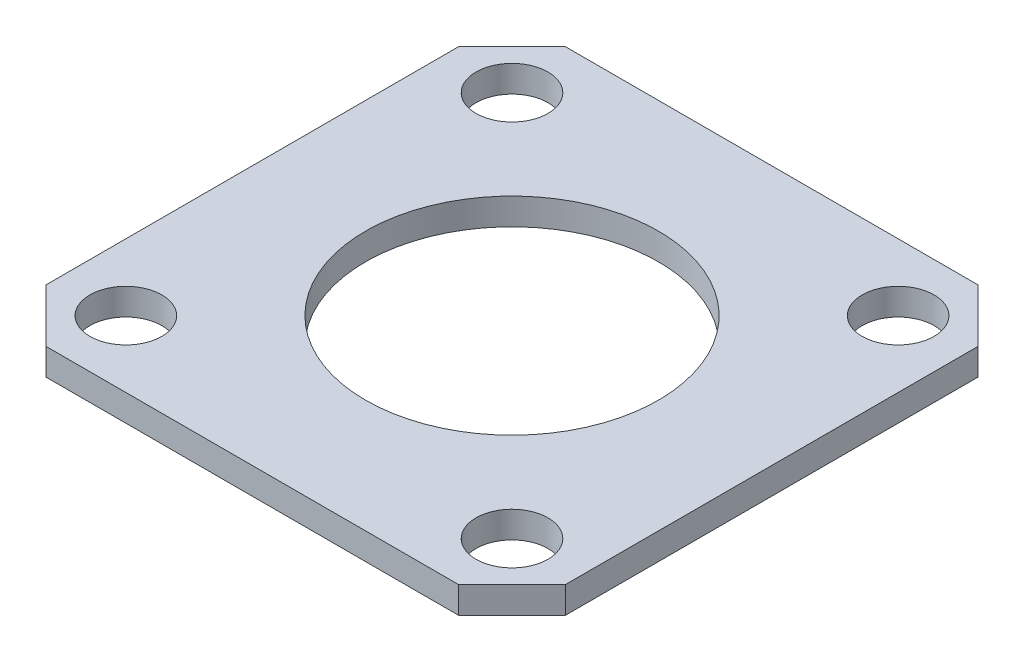
SolidWorks part; units mm, degrees
material "SUS 304"
ref_plane "Front Plane" through (0, 0, 0) normal (0, 0, 1) x (1, 0, 0)
ref_plane "Top Plane" through (0, 0, 0) normal (0, 1, 0) x (1, 0, 0)
ref_plane "Right Plane" through (0, 0, 0) normal (1, 0, 0) x (0, 0, -1)
sketch "Sketch1" plane through (0, 0, 0) normal (0, 1, 0) x (1, 0, 0)
  line L0 (7.75, -9.75) -> (9.75, -7.75)
  line L1 (-7.75, 9.75) -> (7.75, 9.75)
  line L2 (-9.75, 7.75) -> (-9.75, -7.75)
  line L3 (-7.75, -9.75) -> (7.75, -9.75)
  line L4 (9.75, 7.75) -> (9.75, -7.75)
  line L5 (-9.75, 9.75) -> (9.75, -9.75) construction
  line L6 (-9.75, -9.75) -> (9.75, 9.75) construction
  line L7 (-9.75, -7.75) -> (-7.75, -9.75)
  line L8 (-9.75, 7.75) -> (-7.75, 9.75)
  line L9 (7.75, 9.75) -> (9.75, 7.75)
  circle A0 centre (0, 0) radius 5.5
  point P0 (0, 0)
  dimension "D3" = 11
  dimension "D1" = 19.5
  dimension "D2" = 19.5
extrude "Boss-Extrude1" add sketch "Sketch1" along normal blind 1
sketch "Sketch2" plane through (0, 1, 0) normal (0, 1, 0) x (1, 0, 0)
  circle A0 centre (-7.25, 7.25) radius 1.35
  circle A1 centre (0, 0) radius 5.5 construction
  circle A2 centre (7.25, 7.25) radius 1.35
  circle A3 centre (7.25, -7.25) radius 1.35
  circle A4 centre (-7.25, -7.25) radius 1.35
  dimension "D1" = 7.25
  dimension "D2" = 7.25
  dimension "D3" = 2.7
  dimension "D5" = 14.5
  dimension "D4" = 4
extrude "Cut-Extrude1" cut sketch "Sketch2" against normal blind 1
